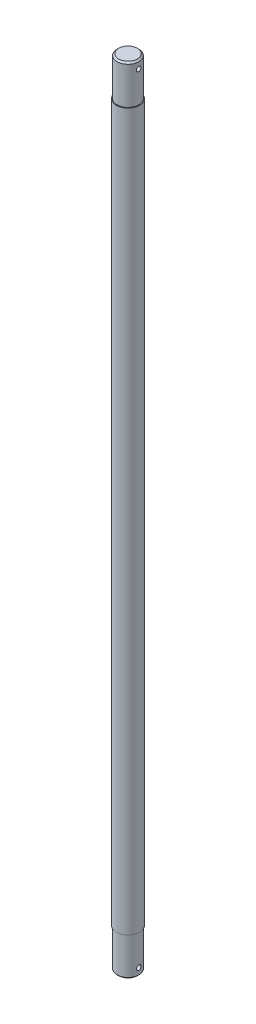
SolidWorks part; units mm, degrees
material "Q235B"
ref_plane "Front Plane" through (0, 0, 0) normal (0, 0, 1) x (1, 0, 0)
ref_plane "Top Plane" through (0, 0, 0) normal (0, 1, 0) x (1, 0, 0)
ref_plane "Right Plane" through (0, 0, 0) normal (1, 0, 0) x (0, 0, -1)
sketch "Sketch1" plane through (0, 0, 0) normal (0, 0, 1) x (1, 0, 0)
  line L0 (0, 0) -> (7, 0)
  line L1 (7, 0) -> (7, 25)
  line L2 (7, 25) -> (7.5, 25)
  line L3 (7.5, 25) -> (7.5, 485)
  line L4 (7.5, 485) -> (7, 485)
  line L5 (7, 485) -> (7, 510)
  line L6 (7, 510) -> (0, 510)
  line L7 (0, 510) -> (0, 0)
  line L8 (0, 0) -> (0, -3.5159) construction
  dimension "D1" = 14
  dimension "D2" = 15
  dimension "D3" = 510
  dimension "D4" = 25
revolve "Revolve1" add sketch "Sketch1" angle 360 about L8
cosmetic thread "Cosmetic Thread1" parameters "D1"=25, "D2"=11.835
cosmetic thread "Cosmetic Thread2" parameters "D1"=25, "D2"=11.835
chamfer "Chamfer1" distance 1 angle 45 2 edges at (0, 0, 7) (0, 510, 7)
sketch "Sketch3" plane through (0, 0, 0) normal (1, 0, 0) x (0, 0, -1)
  line L0 (0, 510) -> (0, 505) construction
  line L1 (6, 510) -> (-6, 510) construction
  line L2 (7.5, 255) -> (58.4347, 255) construction
  line L3 (7.5, 25) -> (7.5, 485) construction
  line L4 (0, 0) -> (0, 5) construction
  circle A0 centre (0, 505) radius 1.5
  circle A1 centre (0, 5) radius 1.5
  dimension "D2" = 3
  dimension "D1" = 5
extrude "Cut-Extrude1" cut sketch "Sketch3" against normal through all both and the other way through all
